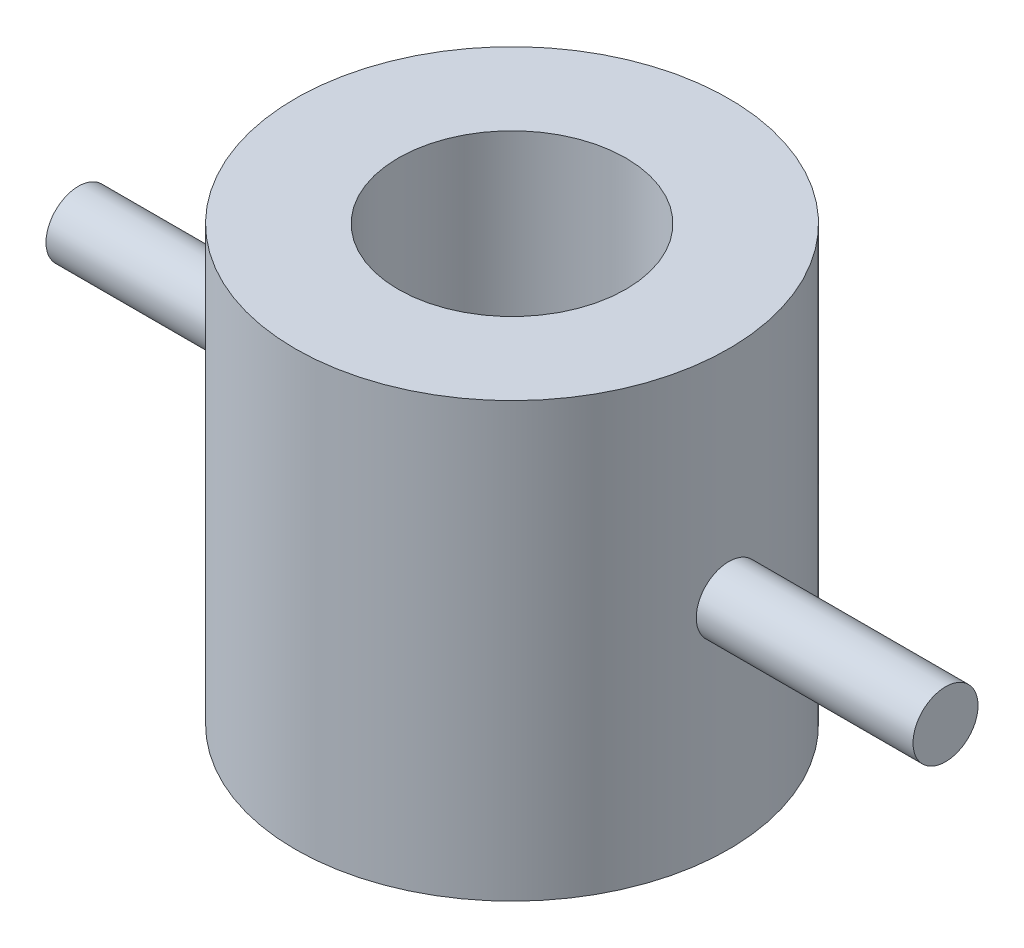
SolidWorks part; units mm, degrees
ref_plane "前视基准面" through (0, 0, 0) normal (0, 0, 1) x (1, 0, 0)
ref_plane "上视基准面" through (0, 0, 0) normal (0, 1, 0) x (1, 0, 0)
ref_plane "右视基准面" through (0, 0, 0) normal (1, 0, 0) x (0, 0, -1)
sketch "草图2" plane through (0, 0, 0) normal (0, 1, 0) x (1, 0, 0)
  circle A0 centre (0, 0) radius 20
  circle A1 centre (0, 0) radius 10.5
  dimension "D1" = 21
  dimension "D2" = 40
extrude "凸台-拉伸1" add sketch "草图2" along normal blind 40
ref_plane "基准面1" through (-20, 0, 0) normal (-1, 0, 0) x (0, 0, 1)
sketch "草图3" plane through (-20, 0, 0) normal (-1, 0, 0) x (0, 0, 1)
  line L0 (0, -22) -> (0, 22) construction
  line L1 (22, 0) -> (-22, 0) construction
  circle A0 centre (0, 20) radius 3
  dimension "D1" = 6
  dimension "D2" = 20
extrude "凸台-拉伸2" add sketch "草图3" along normal blind 20 separate body
mirror "镜向3" about plane through (0, 0, 0) normal (1, 0, 0) of bodies 107
